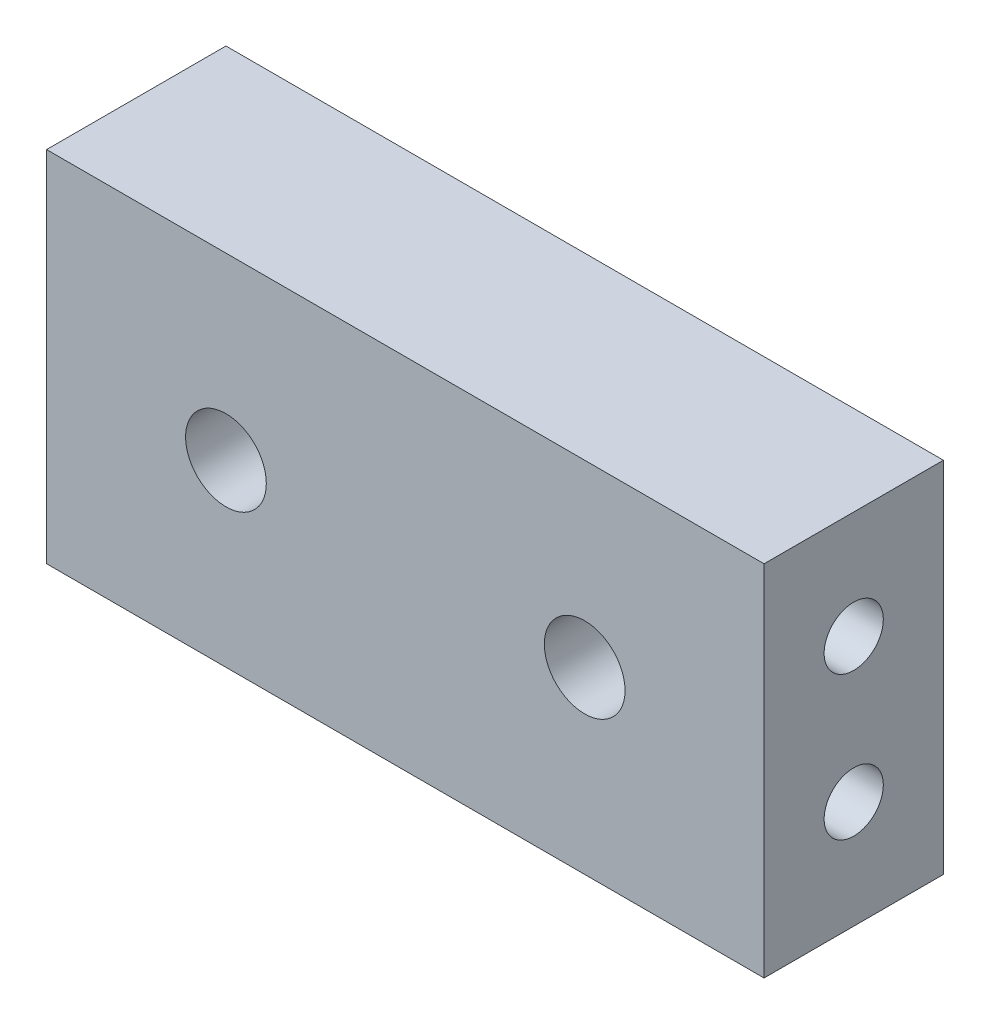
from build123d import *

# Parameters (mm, degrees)
SKETCH_1_W          = 40
SKETCH_1_H          = 20
SKETCH_1_R          = 2.25
EXTRUDE_1_DEPTH     = 10
SKETCH_3_R          = 1.65
CUT_EXTRUDE_1_DEPTH = 11.5
CUT_EXTRUDE_START   = -11.5
SKETCH_4_R          = 1.65
CUT_EXTRUDE_2_DEPTH = 11.5


with BuildPart() as part:
    # 草图1 → 凸台-拉伸1 (new body)
    with BuildSketch(Plane.XY):
        with Locations((0.651465798, 0.195439739)):
            Rectangle(SKETCH_1_W, SKETCH_1_H)
        with Locations((-9.348534202, 0.195439739)):
            Circle(SKETCH_1_R, mode=Mode.SUBTRACT)
        with Locations((10.651465798, 0.195439739)):
            Circle(SKETCH_1_R, mode=Mode.SUBTRACT)
    extrude(amount=EXTRUDE_1_DEPTH)

    # 草图3 → 切除-拉伸1 (cut)
    with BuildSketch(Plane.ZY.offset(19.348534202)):
        with Locations(Location((5, 4.195439739, 0), (0, 0, 270))):
            Circle(SKETCH_3_R)
        with Locations(Location((5, -3.804560261, 0), (0, 0, 270))):
            Circle(SKETCH_3_R)
    extrude(amount=-CUT_EXTRUDE_1_DEPTH, mode=Mode.SUBTRACT)

    # 草图4 → 切除-拉伸2 (cut)
    with BuildSketch(Plane(origin=(20.651465798, 0, 0), x_dir=(0, 0, -1), z_dir=(1, 0, 0)).offset(CUT_EXTRUDE_START)):
        with Locations(Location((-5, 4.195439739, 0), (0, 0, 270))):
            Circle(SKETCH_4_R)
        with Locations(Location((-5, -3.804560261, 0), (0, 0, 270))):
            Circle(SKETCH_4_R)
    extrude(amount=CUT_EXTRUDE_2_DEPTH, mode=Mode.SUBTRACT)


solid = part.part
